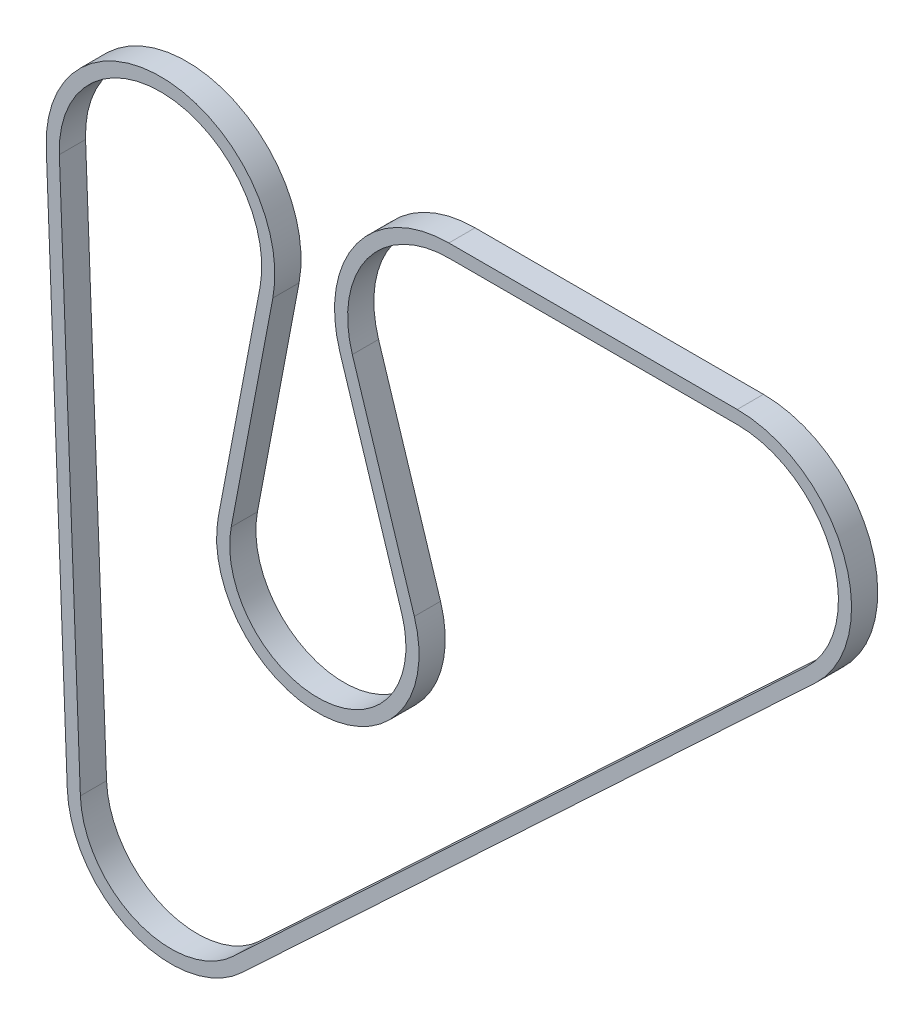
SolidWorks part; units mm, degrees
ref_plane "前视基准面" through (0, 0, 0) normal (0, 0, 1) x (1, 0, 0)
ref_plane "上视基准面" through (0, 0, 0) normal (0, 1, 0) x (1, 0, 0)
ref_plane "右视基准面" through (0, 0, 0) normal (1, 0, 0) x (0, 0, -1)
sketch "草图2" plane through (0, 0, 0) normal (0, 0, 1) x (1, 0, 0)
  line L0 (0, 0) -> (1, 0) construction
  line L1 (0, 0) -> (0, 1) construction
  line L2 (-34.5722, -1.3338) -> (-42.5909, 206.5111)
  line L3 (33.9408, 200.7908) -> (18.0592, 117.2092)
  line L4 (92.8197, 121.6527) -> (69.1803, 196.3473)
  line L5 (106, 246.6196) -> (216, 246.6196)
  line L6 (242.4127, 179.8247) -> (23.6622, -25.2412)
  arc A0 (23.6622, -25.2412) -> (-34.5722, -1.3338) centre (0, 0) cw
  arc A1 (-42.5909, 206.5111) -> (33.9408, 200.7908) centre (-4, 208) cw
  arc A2 (18.0592, 117.2092) -> (92.8197, 121.6527) centre (56, 110) ccw
  arc A3 (69.1803, 196.3473) -> (106, 246.6196) centre (106, 208) cw
  arc A4 (216, 246.6196) -> (242.4127, 179.8247) centre (216, 208) cw
extrude "拉伸-薄壁1" add sketch "草图2" along normal blind 10 thin thin type one direction wall 5
